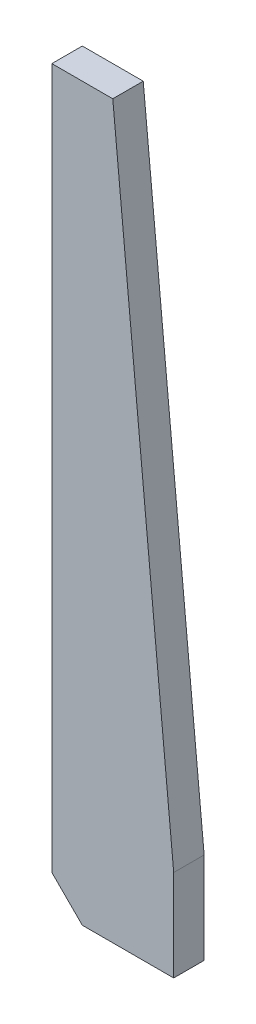
from build123d import *

# Parameters (mm, degrees)
EXTRUDE_1_DEPTH = 5
CHAMFER_1_SIZE  = 5


with BuildPart() as part:
    # 草图1 → 凸台-拉伸1 (new body)
    with BuildSketch(Plane.XY):
        Polygon((0, 0), (0, 120), (10, 120), (20, 15), (20, 0), align=None)
    extrude(amount=EXTRUDE_1_DEPTH)

    # 倒角1
    chamfer_1_edges = [part.edges().sort_by_distance(p)[0] for p in [
        (0, 0, 2.5),
    ]]
    chamfer(chamfer_1_edges, length=CHAMFER_1_SIZE)


solid = part.part
